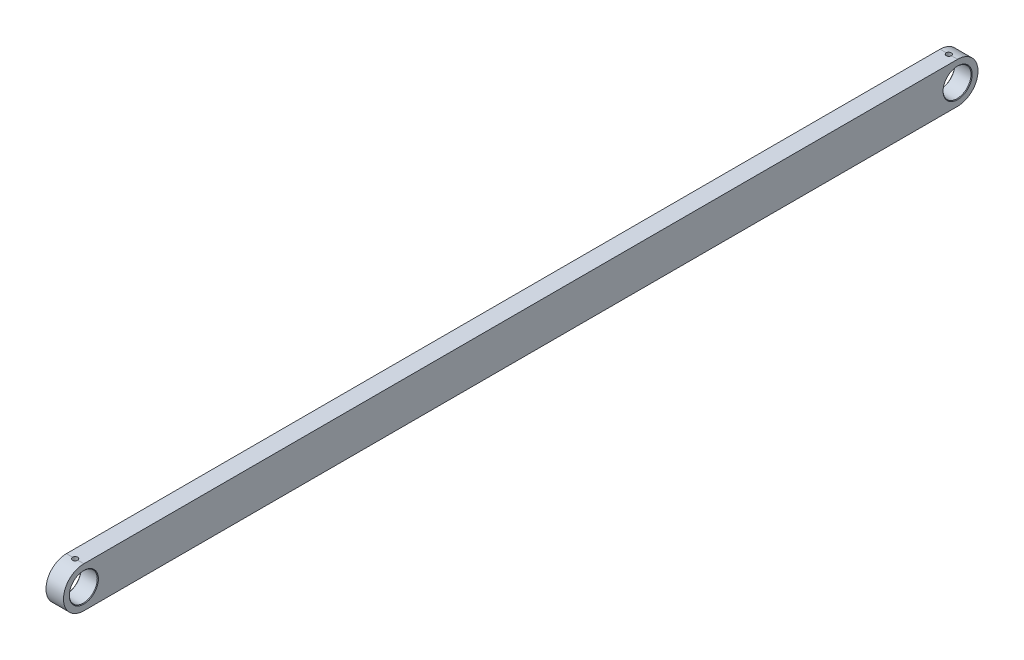
from build123d import *

# Parameters (mm, degrees)
SKETCH_1_R      = 24
EXTRUDE_1_DEPTH = 15
M10X1_0_1_D     = 9
M10X1_0_1_DEPTH = 20
M10X1_0_1_TIP   = 2.703872786
CHAMFER_1_SIZE  = 1


with BuildPart() as part:
    # 草图1 → 凸台-拉伸1 (new, symmetric)
    with BuildSketch(Plane(origin=(0, 0, 0), x_dir=(0, 0, -1), z_dir=(1, 0, 0))):
        with BuildLine():
            Line((-750, -35), (750, -35))
            ThreePointArc((750, -35), (785, 0), (750, 35))
            Line((750, 35), (-750, 35))
            ThreePointArc((-750, 35), (-785, 0), (-750, -35))
        make_face()
        with Locations((-750, 0)):
            Circle(SKETCH_1_R, mode=Mode.SUBTRACT)
        with Locations((750, 0)):
            Circle(SKETCH_1_R, mode=Mode.SUBTRACT)
    extrude(amount=EXTRUDE_1_DEPTH, both=True)

    # M10x1.0 螺纹孔1
    with Locations(Plane(origin=(0, 35, 0), x_dir=(1, 0, 0), z_dir=(0, 1, 0))):
        with Locations((0, -750), (0, 750)):
            Hole(M10X1_0_1_D / 2, depth=M10X1_0_1_DEPTH)
            with Locations((0, 0, -(M10X1_0_1_DEPTH + M10X1_0_1_TIP / 2))):  # 118° drill point
                Cone(0, M10X1_0_1_D / 2, M10X1_0_1_TIP, mode=Mode.SUBTRACT)

    # 倒角1
    chamfer_1_edges = [part.edges().sort_by_distance(p)[0] for p in [
        (-15, 0, 774),
        (15, 0, 774),
        (-15, 0, -726),
        (15, 0, -726),
    ]]
    chamfer(chamfer_1_edges, length=CHAMFER_1_SIZE)


solid = part.part
